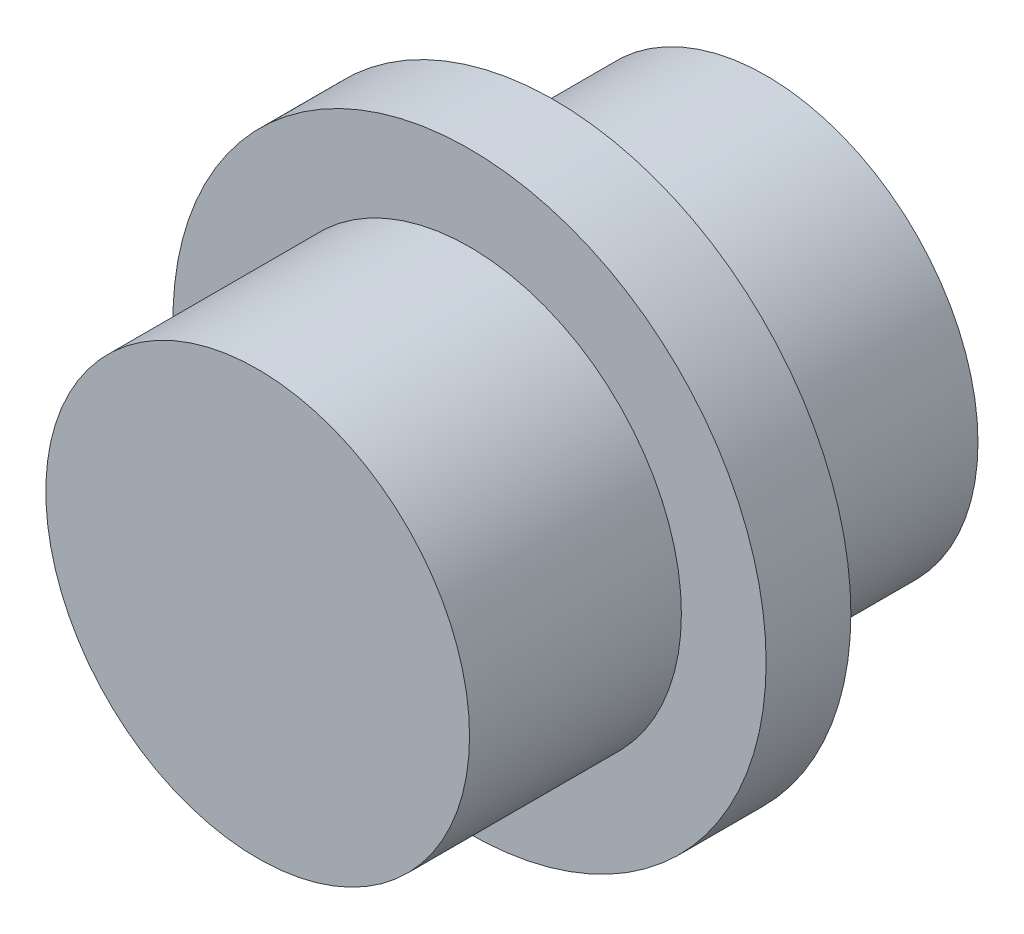
SolidWorks part; units mm, degrees
ref_plane "Front Plane" through (0, 0, 0) normal (0, 0, 1) x (1, 0, 0)
ref_plane "Top Plane" through (0, 0, 0) normal (0, 1, 0) x (1, 0, 0)
ref_plane "Right Plane" through (0, 0, 0) normal (1, 0, 0) x (0, 0, -1)
sketch "Sketch1" plane through (0, 0, 0) normal (0, 0, 1) x (1, 0, 0)
  circle A0 centre (0, 0) radius 5
  dimension "D1" = 10
extrude "Boss-Extrude1" add sketch "Sketch1" along normal blind 5
sketch "Sketch2" plane through (0, 0, 5) normal (0, 0, 1) x (1, 0, 0)
  circle A0 centre (0, 0) radius 7
  dimension "D1" = 14
extrude "Boss-Extrude2" add sketch "Sketch2" along normal blind 2
sketch "Sketch4" plane through (0, 0, 7) normal (0, 0, 1) x (1, 0, 0)
  circle A0 centre (0, 0) radius 5
  dimension "D1" = 10
extrude "Boss-Extrude3" add sketch "Sketch4" along normal blind 5
